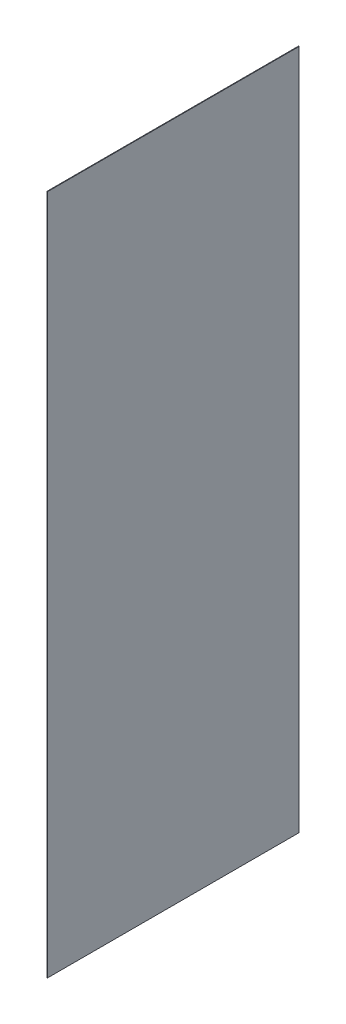
SolidWorks part; units mm, degrees
ref_plane "Front Plane" through (0, 0, 0) normal (0, 0, 1) x (1, 0, 0)
ref_plane "Top Plane" through (0, 0, 0) normal (0, 1, 0) x (1, 0, 0)
ref_plane "Right Plane" through (0, 0, 0) normal (1, 0, 0) x (0, 0, -1)
other "Configuration Table"
sketch "Sketch1" plane through (-95, 0, 0) normal (-1, 0, 0) x (0, 0, 1)
  line L0 (-1057, 2872) -> (1057, 2872) construction
  line L1 (-1062, -2872) -> (1062, -2872)
  line L2 (-1062, -2872) -> (-1062, 2872)
  line L3 (-1062, 2872) -> (1062, 2872)
  line L4 (1062, -2872) -> (1062, 2872)
  line L5 (-1062, -2872) -> (1062, 2872) construction
  line L6 (-1062, 2872) -> (1062, -2872) construction
  line L7 (-1062, 2851) -> (-1062, -2851) construction
  point P0 (0, 0)
extrude "Boss-Extrude1" add sketch "Sketch1" along normal blind 5
